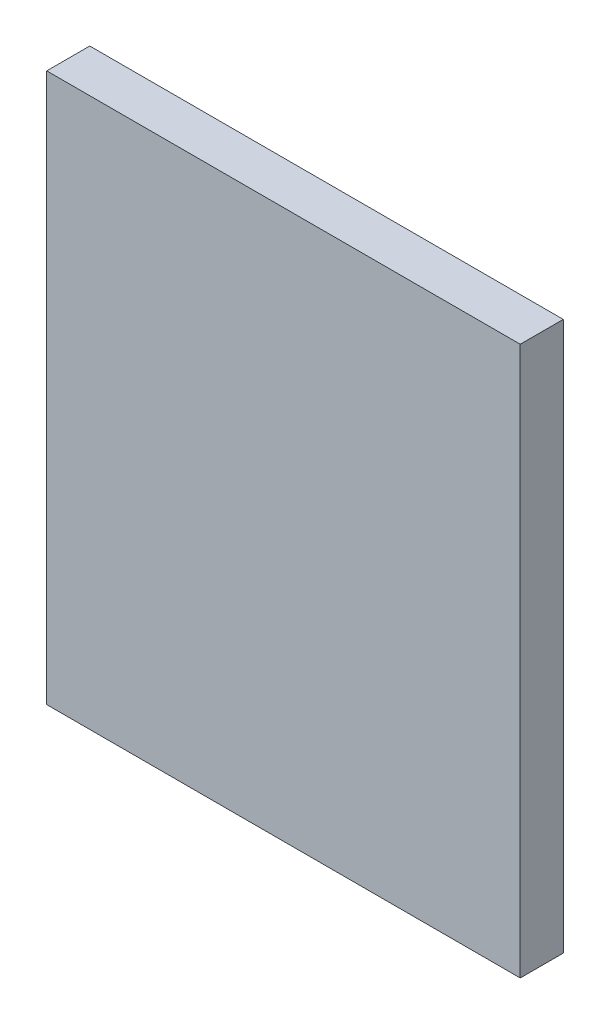
from build123d import *

# Parameters (mm, degrees)
SKETCH1_W           = 440
SKETCH1_H           = 510
BOSS_EXTRUDE1_DEPTH = 40


with BuildPart() as part:
    # Sketch1 → Boss-Extrude1 (new body)
    with BuildSketch(Plane.XY):
        with Locations((220, 255)):
            Rectangle(SKETCH1_W, SKETCH1_H)
    extrude(amount=BOSS_EXTRUDE1_DEPTH)


solid = part.part
